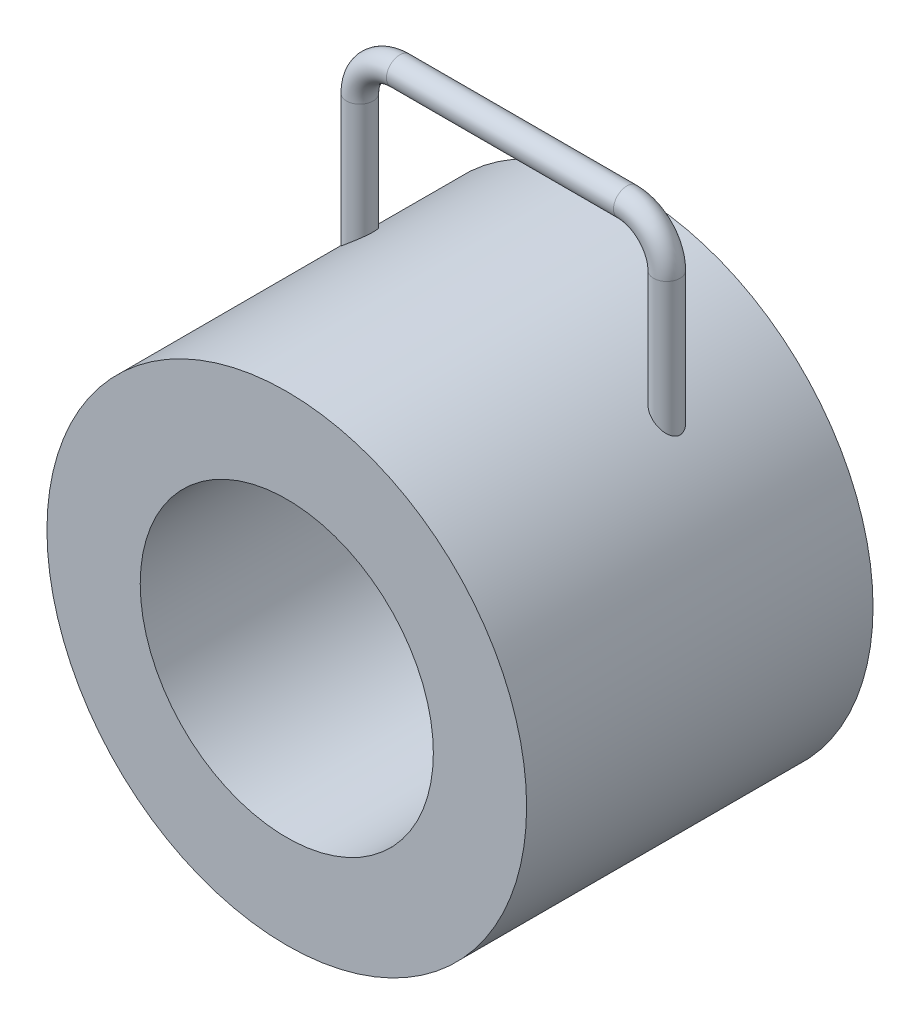
SolidWorks part; units mm, degrees
ref_plane "Front Plane" through (0, 0, 0) normal (0, 0, 1) x (1, 0, 0)
ref_plane "Top Plane" through (0, 0, 0) normal (0, 1, 0) x (1, 0, 0)
ref_plane "Right Plane" through (0, 0, 0) normal (1, 0, 0) x (0, 0, -1)
sketch "Sketch1" plane through (0, 0, 0) normal (0, 0, 1) x (1, 0, 0)
  circle A0 centre (0, 0) radius 90
  dimension "D1" = 180
extrude "Boss-Extrude1" add sketch "Sketch1" along normal blind 130
sketch "Sketch2" plane through (0, 0, 130) normal (0, 0, 1) x (1, 0, 0)
  circle A0 centre (0, 0) radius 55
  dimension "D1" = 110
extrude "Cut-Extrude1" cut sketch "Sketch2" against normal blind 100
ref_plane "Plane1" through (0, 0, 45) normal (0, 0, -1) x (-1, 0, 0)
sketch "Sketch3" plane through (0, 0, 45) normal (0, 0, -1) x (-1, 0, 0)
  line L0 (-57.6, 56.7892) -> (-57.6, 115.5892)
  line L1 (-42.6, 130.5892) -> (42.6, 130.5892)
  line L2 (57.6, 115.5892) -> (57.6, 56.7892)
  line L3 (0, 0) -> (0, 50.3545) construction
  arc A0 (42.6, 130.5892) -> (57.6, 115.5892) centre (42.6, 115.5892) cw
  arc A1 (-57.6, 115.5892) -> (-42.6, 130.5892) centre (-42.6, 115.5892) cw
  point P12 (57.6, 130.5892)
  dimension "D2" = 15
  dimension "D1" = 57.6
  dimension "D3" = 73.8
sweep "Sweep1" add path "Sketch3" circular profile diameter 10 parameters "D3"=10
